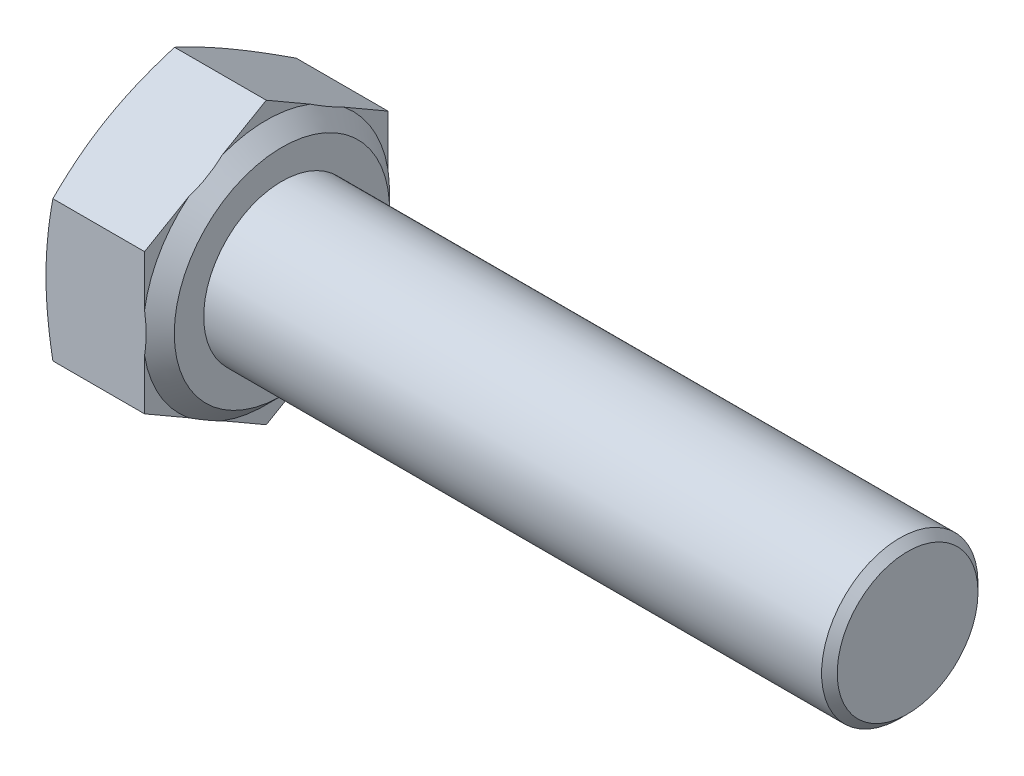
from build123d import *

# Parameters (mm, degrees)
BASEHEAD_DEPTH = 3.65
SKETCH5_R      = 2.5
BASEBODY_DEPTH = 20
CHAMFER1_SIZE  = 0.25


with BuildPart() as part:
    # Sketch2 → BaseHead (new body)
    with BuildSketch(Plane(origin=(0, 0, 0), x_dir=(0, 0, -1), z_dir=(1, 0, 0))):
        Polygon((3.89, -2.245892547), (3.89, 2.245892547), (0, 4.491785094), (-3.89, 2.245892547), (-3.89, -2.245892547), (0, -4.491785094), align=None)
    extrude(amount=BASEHEAD_DEPTH)

    # Sketch3 → BearingFace (revolve, cut)
    with BuildSketch(Plane.XY, mode=Mode.PRIVATE) as bearingface_sk:
        Polygon((3.65, 4.491785094), (3.65, 3.44), (3.15, 3.94), (3.15, 4.491785094), align=None)
    revolve(bearingface_sk.sketch.rotate(Axis((-0.957090588, 0, 0), (1, 0, 0)), 90), axis=Axis((-0.957090588, 0, 0), (1, 0, 0)), mode=Mode.SUBTRACT)

    # Sketch4 → HeadChamfer (revolve, cut)
    with BuildSketch(Plane.XY):
        Polygon((0, 4.491785094), (0.219031862, 4.491785094), (0, 3.89), align=None)
    revolve(axis=Axis((-0.493528746, 0, 0), (1, 0, 0)), mode=Mode.SUBTRACT)

    # Sketch5 → BaseBody (add)
    with BuildSketch(Plane(origin=(3.65, 0, 0), x_dir=(0, 0, -1), z_dir=(1, 0, 0))):
        Circle(SKETCH5_R)
    extrude(amount=BASEBODY_DEPTH)

    # Chamfer1
    chamfer1_edges = [part.edges().sort_by_distance(p)[0] for p in [
        (23.65, 0, 2.5),
    ]]
    chamfer(chamfer1_edges, length=CHAMFER1_SIZE)


solid = part.part
